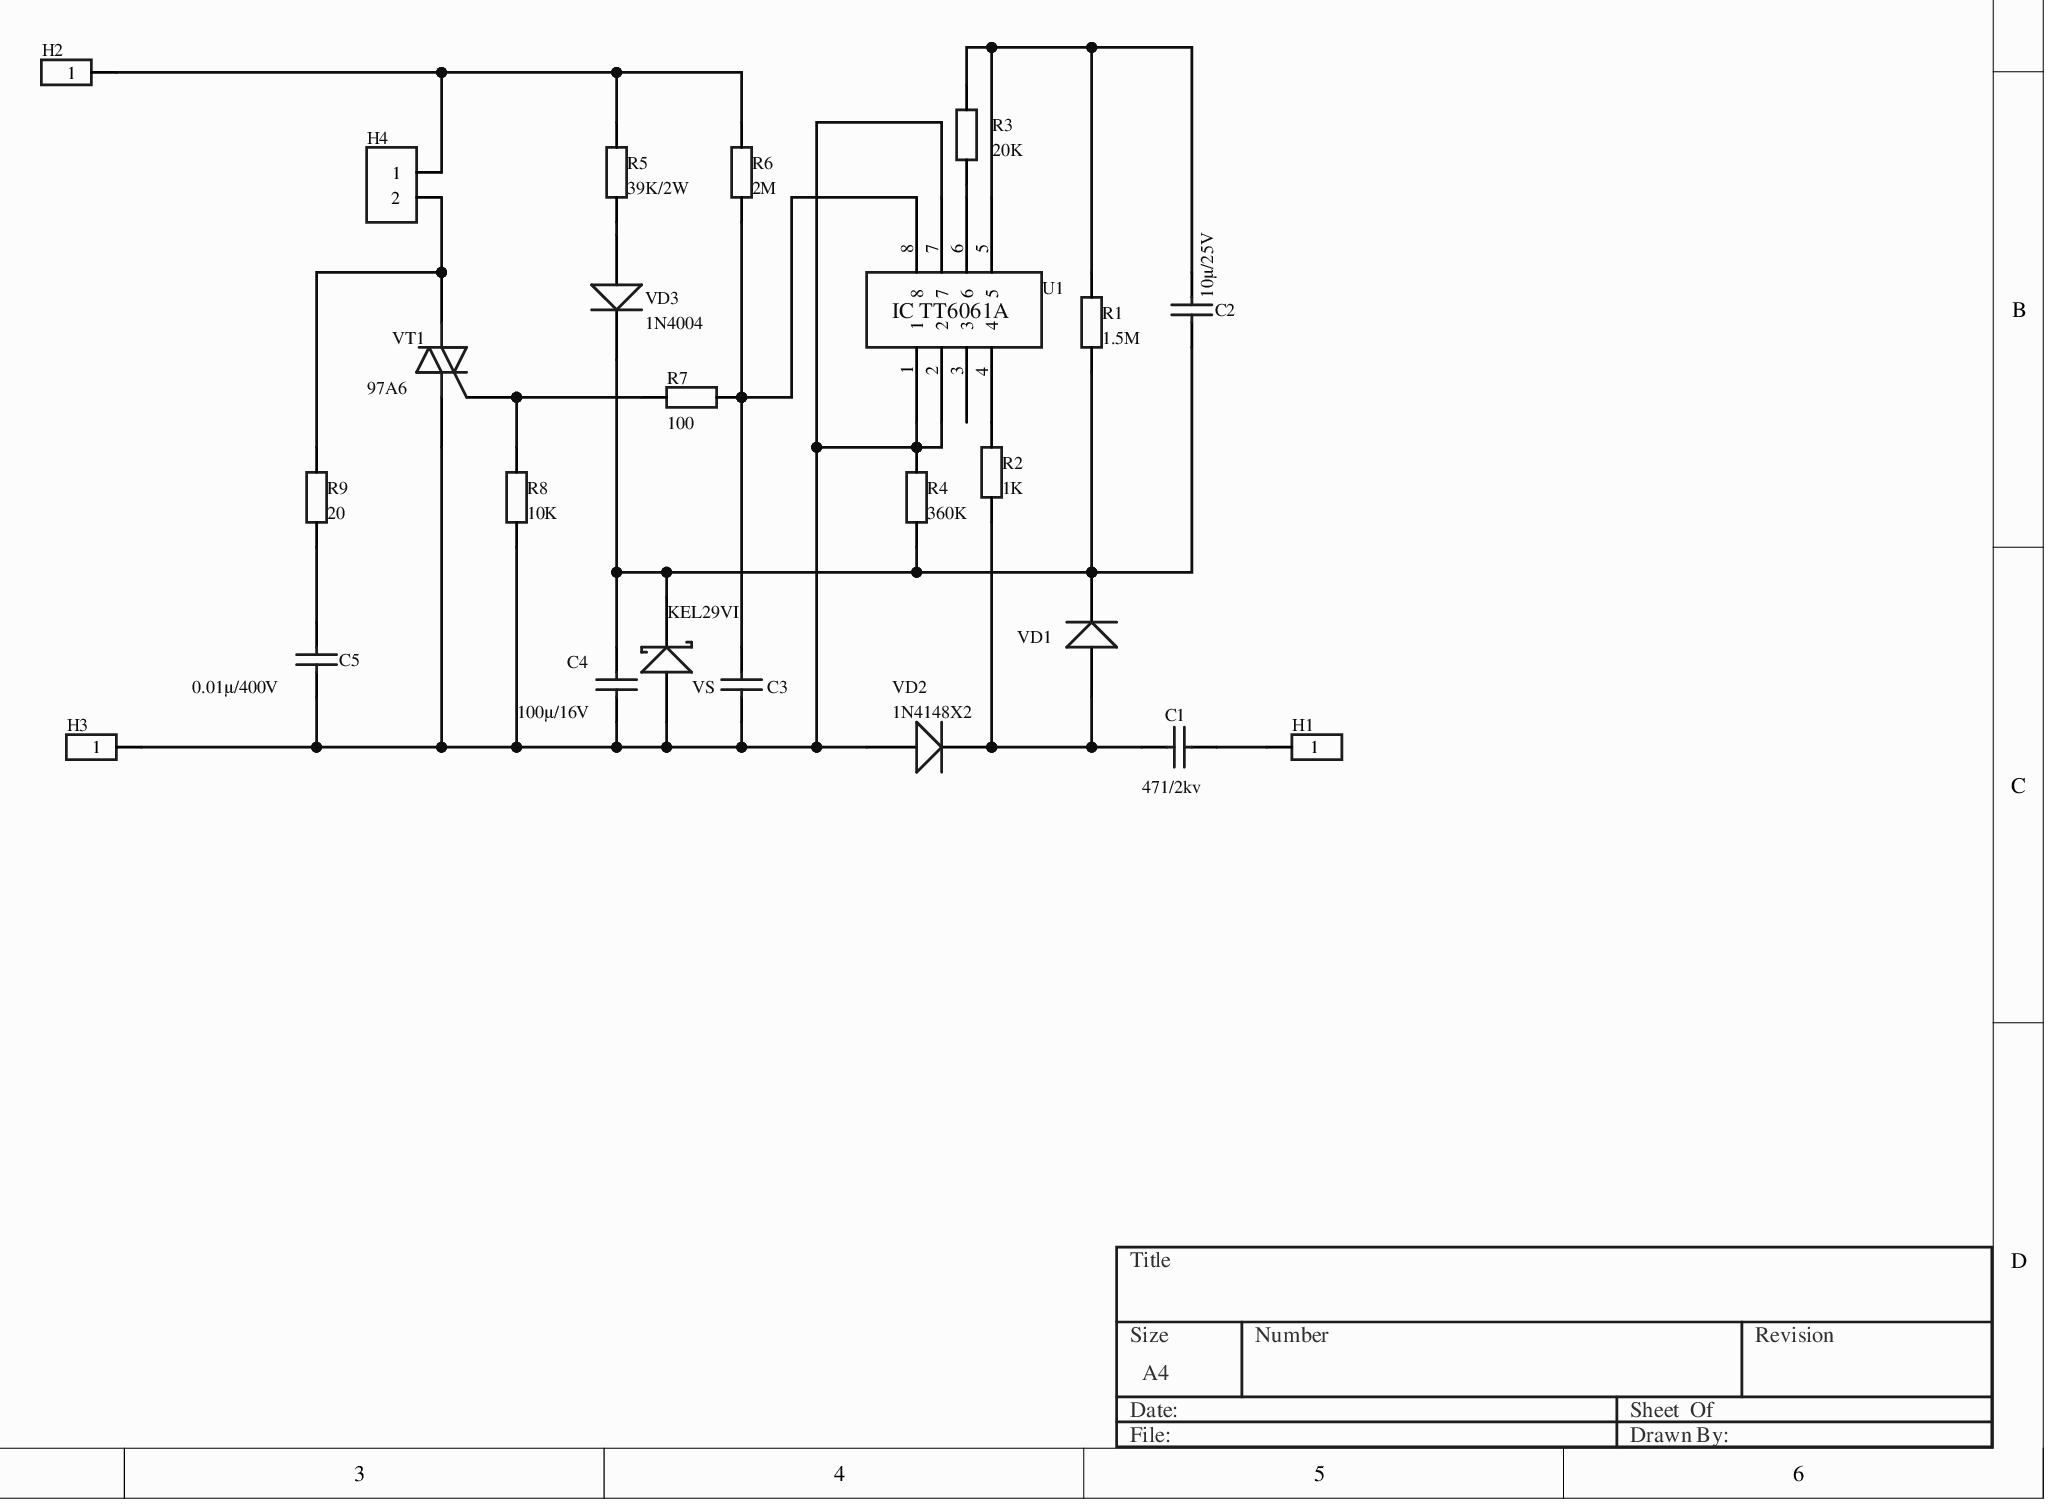
[diagram p0: MISC75395-3.schdoc]
# Altium project MISC75395-2.PrjPcb
1 sheet, 24 parts. Net scope: global (net labels, ports and power ports of the same name join across sheets).
Board file: MISC75395.pcbdoc

## Sheet MISC75395-3.schdoc
size 292 x 193 mm; @Page No: 1; @Page Count: 1; @Schematic Name: MISC75395; @Project Name: MISC75395; @Board Name: MISC75395; @Update Date: 2025-05-19; @Create Time: 21:32:10; @Update Time: 21:45:53; @Create Date: 2025-05-19

### Parts
C1  value 471/2kv  [RAD-0.3]
C2  value 10μ/25V  [RAD-0.3]
C3  (no value)  [RAD-0.3]
C4  value 100μ/16V  [RAD-0.3]
C5  value 0.01μ/400V  [RAD-0.3]
H1  (no value)  [HDR-TH_1P-V-M_XKB_X4611WV-01I-C28D40]
H2  (no value)  [HDR-TH_1P-V-M_XKB_X4611WV-01I-C28D40]
H3  (no value)  [HDR-TH_1P-V-M_XKB_X4611WV-01I-C28D40]
H4  (no value)  [HDR-TH_2P-P2.54-V-F]
R1  1.5M  [Res_1/4W]
R2  1K  [Res_1/4W]
R3  20K  [Res_1/4W]
R4  360K  [Res_1/4W]
R5  39K/2W  [Res_1/4W]
R6  2M  [Res_1/4W]
R7  100  [Res_1/4W]
R8  10K  [Res_1/4W]
R9  20  [Res_1/4W]
U1  (no value)  [DIP-8_L9.2-W6.6-P2.54-LS7.62-BL]
VD1  (no value)  [DO-41_BD2.4-L4.7-P8.70-D0.9-RD]
VD2  1N4148X2  [DO-41_BD2.4-L4.7-P8.70-D0.9-RD]
VD3  1N4004  [DO-41_BD2.4-L4.7-P8.70-D0.9-RD]
VS  KEL29VI  [DO-41_BD2.4-L4.7-P8.70-D0.9-RD]
VT1  97A6  [SOT-23-3_L2.9-W1.6-P1.90-LS2.8-BR]

### Nets
NetC1_1: C1.1 R2.1 VD1.1 VD2.3
NetC1_2: C1.2 H1.1
NetC2_1: C2.1 C4.2 R1.1 R4.1 VD1.3 VD3.3 VS.1
NetC2_2: C2.2 R1.2 R3.2 U1.5
NetC3_1: C3.1 C4.1 C5.1 H3.1 R4.2 R8.1 U1.1 U1.2 U1.7 VD2.1 VS.3 VT1.1(M1)
NetC3_2: C3.2 R6.1 R7.1 U1.8
NetC5_2: C5.2 R9.1
NetH2_1: H2.1 H4.1 R5.2 R6.2
NetH4_2: H4.2 R9.2 VT1.2(M2)
NetR2_2: R2.2 U1.4
NetR3_1: R3.1 U1.6
NetR5_1: R5.1 VD3.1
NetR7_2: R7.2 R8.2 VT1.3(G)

Not connected (* = marked no-connect by the designer): U1 3*

### Notes on the sheet
- Title
- File:
- Date:
- Size
- A4
- Number
- Drawn By:
- Sheet
- Of
- Revision

### Library data of the parts
C1-C5 = Cap: Capacitor; AddInBom: yes; Origin Footprint: RAD-0.3; Device: Cap; Symbol: Cap; Design Item ID: Cap; Library Name: Miscellaneous Devices; Published: 8-Jun-2000; LatestRevisionDate: 17-Jul-2002; LatestRevisionNote: Re-released for DXP Platform.; PackageReference: RAD-0.3; PackageDescription: Radial Cap, Thru-Hole; 2 Leads; 0.3 in Pin Spacing; FootprintName: RAD-0.3; ConvertToPcb: yes; Publisher: Altium Limited
H1-H3 = HDR-M_2.54_1x1P: Symbol: HDR_1x1; ConvertToPcb: yes; ModelId: 95857080d3cc4057a19a22ccce05e171; ModelTransform: 78.74,79.1337,0,0,0,0,0,0,-110.236; Device: HDR-M_2.54_1x1P; AddInBom: yes; SupplierPart: C81276; Supplier Footprint: 插件; FootprintName: HDR-TH_1P-V-M_XKB_X4611WV-01I-C28D40; JLCPCB Part Class: Extended Part; ModelName: HDR-TH_1P-V-M_XKB_X4611WV-01I-C28D40
H4 = HDR-F_2.54_1x2P: Symbol: Header-Female-2.54_1x2; ConvertToPcb: yes; ModelId: a9450ef445564560a104363b9aacde4e; ModelName: HDR-TH_2P-P2.54-F-LI-1X2P; ModelTransform: 215.7476,98.425,0,0,0,0,0,0,-129.921; Device: HDR-F_2.54_1x2P; AddInBom: yes; SupplierPart: C49661; Supplier Footprint: 插件; FootprintName: HDR-TH_2P-P2.54-V-F
R1 = 1.5M: Resistor; Origin Footprint: AXIAL-0.4; Symbol: Res2; AddInBom: yes; Device: 1.5M; Design Item ID: Res2; Library Name: Miscellaneous Devices; Published: 8-Jun-2000; LatestRevisionDate: 17-Jul-2002; LatestRevisionNote: Re-released for DXP Platform.; PackageReference: AXIAL-0.4; PackageDescription: Axial Device, Thru-Hole; 2 Leads; 0.4 in Pin Spacing; ConvertToPcb: yes; Publisher: Altium Limited
R2 = 1K: Resistor; Origin Footprint: AXIAL-0.4; Symbol: Res2; AddInBom: yes; Device: 1K; Design Item ID: Res2; Library Name: Miscellaneous Devices; Published: 8-Jun-2000; LatestRevisionDate: 17-Jul-2002; LatestRevisionNote: Re-released for DXP Platform.; PackageReference: AXIAL-0.4; PackageDescription: Axial Device, Thru-Hole; 2 Leads; 0.4 in Pin Spacing; ConvertToPcb: yes; Publisher: Altium Limited
R3 = 20K: Resistor; Origin Footprint: AXIAL-0.4; Symbol: Res2; AddInBom: yes; Device: 20K; Design Item ID: Res2; Library Name: Miscellaneous Devices; Published: 8-Jun-2000; LatestRevisionDate: 17-Jul-2002; LatestRevisionNote: Re-released for DXP Platform.; PackageReference: AXIAL-0.4; PackageDescription: Axial Device, Thru-Hole; 2 Leads; 0.4 in Pin Spacing; ConvertToPcb: yes; Publisher: Altium Limited
R4 R7 = 360K: Resistor; Origin Footprint: AXIAL-0.4; Symbol: Res2; AddInBom: yes; Device: 360K; Design Item ID: Res2; Library Name: Miscellaneous Devices; Published: 8-Jun-2000; LatestRevisionDate: 17-Jul-2002; LatestRevisionNote: Re-released for DXP Platform.; PackageReference: AXIAL-0.4; PackageDescription: Axial Device, Thru-Hole; 2 Leads; 0.4 in Pin Spacing; ConvertToPcb: yes; Publisher: Altium Limited
R5 R6 R8 = 10K: Resistor; Origin Footprint: AXIAL-0.4; Symbol: Res2; AddInBom: yes; Device: 10K; Design Item ID: Res2; Library Name: Miscellaneous Devices; Published: 8-Jun-2000; LatestRevisionDate: 17-Jul-2002; LatestRevisionNote: Re-released for DXP Platform.; PackageReference: AXIAL-0.4; PackageDescription: Axial Device, Thru-Hole; 2 Leads; 0.4 in Pin Spacing; ConvertToPcb: yes; Publisher: Altium Limited
R9 = 20: Resistor; Origin Footprint: AXIAL-0.4; Symbol: Res2; AddInBom: yes; Device: 20; Design Item ID: Res2; Library Name: Miscellaneous Devices; Published: 8-Jun-2000; LatestRevisionDate: 17-Jul-2002; LatestRevisionNote: Re-released for DXP Platform.; PackageReference: AXIAL-0.4; PackageDescription: Axial Device, Thru-Hole; 2 Leads; 0.4 in Pin Spacing; ConvertToPcb: yes; Publisher: Altium Limited
U1 = Component_1: AddInBom: yes; Origin Footprint: Component_1; Device: Component_1; Symbol: Component_1; Design Item ID: Component_1; Library Name: Schlib1; ConvertToPcb: yes
VD1 = Diode BAS116: Silicon Low Leakage Diode; Origin Footprint 1: SOT-23_N; Note: Pin 2 is not connected and not drawn.; Origin Footprint 2: SOT-23_L; Origin Footprint 3: SOT-23_M; AddInBom: yes; Device: Diode BAS116; Symbol: Diode BAS116; Design Item ID: Diode BAS116; Library Name: Miscellaneous Devices; Published: 21-Mar-2003; LatestRevisionDate: 29-May-2009; LatestRevisionNote: IPC-7351 Footprint Added.; DatasheetVersion: Oct-1999; PackageVersion: Sep-2001; PackageReference: SOT-23; PackageDescription: 3-Pin SOT-23 Package 0.95 mm Pitch, 2.5 mm Lead Span; ComponentLink1Description: Manufacturer Link; Datasheet: example.com/upload/Document/cmc_upload/documents/080/656/bas116series.pdf; ComponentLink2Description: Datasheet; ComponentLink2URL: example.com/upload/Document/cmc_upload/documents/080/656/bas116series.pdf; ConvertToPcb: yes; Publisher: Altium Limited
VD2 VD3 = 1N4148X2: Silicon Low Leakage Diode; Origin Footprint 1: SOT-23_N; Symbol: Diode BAS116; Note: Pin 2 is not connected and not drawn.; Origin Footprint 2: SOT-23_L; Origin Footprint 3: SOT-23_M; AddInBom: yes; Device: 1N4148X2; Design Item ID: Diode BAS116; Library Name: Miscellaneous Devices; Published: 21-Mar-2003; LatestRevisionDate: 29-May-2009; LatestRevisionNote: IPC-7351 Footprint Added.; DatasheetVersion: Oct-1999; PackageVersion: Sep-2001; PackageReference: SOT-23; PackageDescription: 3-Pin SOT-23 Package 0.95 mm Pitch, 2.5 mm Lead Span; ComponentLink1Description: Manufacturer Link; Datasheet: example.com/upload/Document/cmc_upload/documents/080/656/bas116series.pdf; ComponentLink2Description: Datasheet; ComponentLink2URL: example.com/upload/Document/cmc_upload/documents/080/656/bas116series.pdf; ConvertToPcb: yes; Publisher: Altium Limited
VS = KEL29VI: Schottky Rectifier; Origin Footprint: TO-220AC; Symbol: Diode 18TQ045; Note: Terminal 2 is the TAB and is electrically connected to the cathode; AddInBom: yes; Device: KEL29VI; Design Item ID: Diode 18TQ045; Library Name: Miscellaneous Devices; Published: 8-Jun-2000; LatestRevisionDate: 17-Jul-2002; LatestRevisionNote: Re-released for DXP Platform.; DatasheetVersion: Dec-1997; PackageVersion: Feb-1998; PackageReference: TO-220AC; PackageDescription: TO, Thru-Hole, Vertical, Heatsink Mounted; 3 In-Line Leads (1 Absent); Pitch 2.54 mm; ComponentLink1Description: Manufacturer Link; Datasheet: example.com/product-info/datasheets/data/18tq.pdf; ComponentLink2Description: Datasheet; ComponentLink2URL: example.com/product-info/datasheets/data/18tq.pdf; ConvertToPcb: yes; Publisher: Altium Limited
VT1 = 97A6: Silicon Bidirectional Triode Thyristor; Origin Footprint: 369-03; Symbol: Triac; Note: Pin 2 is electrically connected to Pin 4 (TAB); AddInBom: yes; Device: 97A6; Design Item ID: Triac; Library Name: Miscellaneous Devices; Published: 29-Sep-2000; LatestRevisionDate: 17-Jul-2002; LatestRevisionNote: Re-released for DXP Platform.; DatasheetVersion: 1999; PackageReference: 369-03; PackageDescription: TO, Thru-Hole, Vertical, Heatsink Mounted; 3 In-Line Leads; Pitch 2.28 mm; ComponentLink1Description: Manufacturer Link; ConvertToPcb: yes; Publisher: Altium Limited